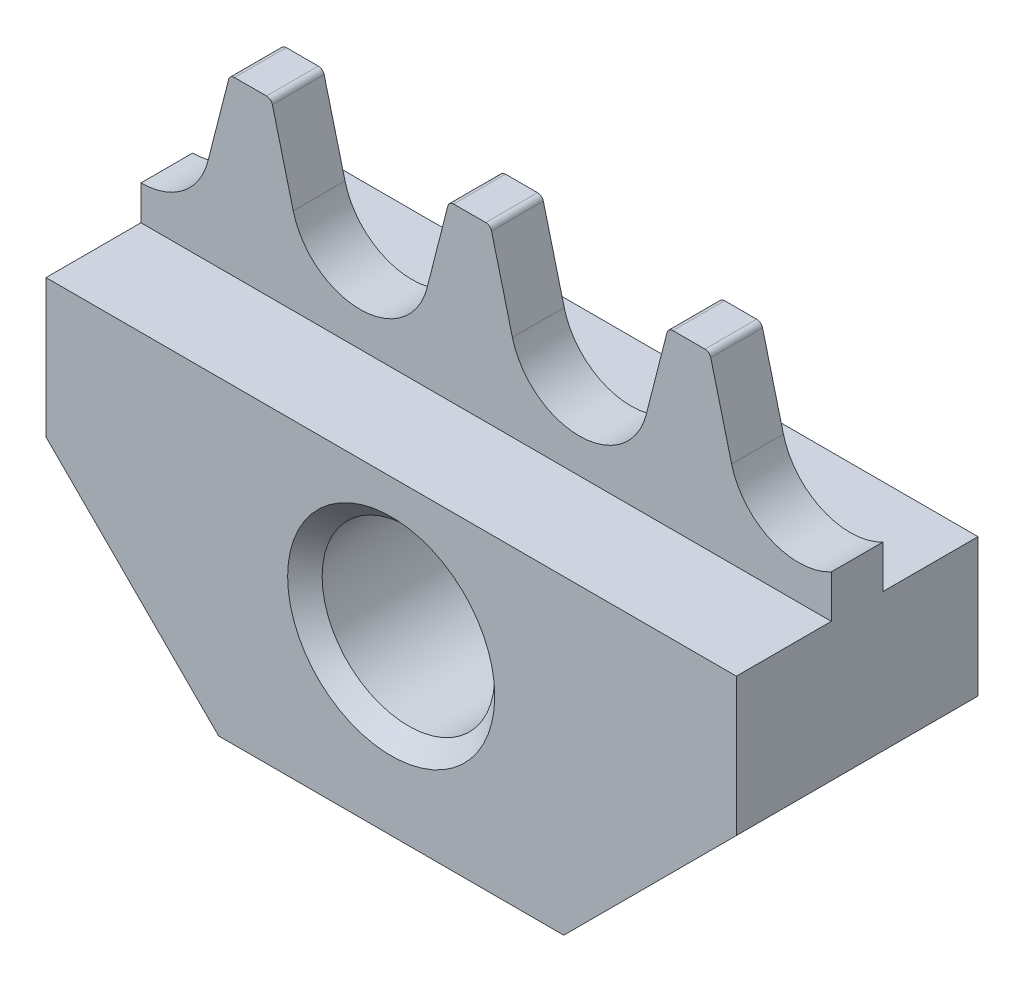
SolidWorks part; units mm, degrees
material "45"
ref_plane "前视基准面" through (0, 0, 0) normal (0, 0, 1) x (1, 0, 0)
ref_plane "上视基准面" through (0, 0, 0) normal (0, 1, 0) x (1, 0, 0)
ref_plane "右视基准面" through (0, 0, 0) normal (1, 0, 0) x (0, 0, -1)
sketch "草图1" plane through (0, 0, 0) normal (0, 0, 1) x (1, 0, 0)
  line L0 (0, 0) -> (0, 18) construction
  line L1 (20, 18) -> (-20, 18)
  line L2 (-20, 18) -> (-20, 10)
  line L4 (10, 0) -> (-10, 0)
  line L5 (-10, 0) -> (-20, 10)
  line L6 (10, 0) -> (20, 10)
  line L7 (20, 18) -> (20, 10)
  circle A0 centre (0, 10) radius 5
  dimension "D5" = 10
  dimension "D1" = 8
  dimension "D2" = 20
  dimension "D3" = 40
  dimension "D4" = 10
extrude "凸台-拉伸1" add sketch "草图1" along normal mid plane 14
sketch "草图2" plane through (0, 0, 0) normal (0, 0, 1) x (1, 0, 0)
  line L0 (-14.85, 28) -> (-12.45, 28)
  line L1 (-10, 0) -> (10, 0) construction
  line L2 (-20, 18) -> (-20, 10) construction
  line L3 (-35.3045, 24) -> (22.0082, 24) construction
  line L4 (-20, 24) -> (-7.3, 24) construction
  line L5 (-20, 18) -> (-20, 20)
  line L6 (-20, 18) -> (20, 18)
  line L7 (-14.85, 28) -> (-16.1244, 23.0102)
  line L8 (-13.65, 28) -> (-13.65, 18) construction
  line L9 (-12.45, 28) -> (-11.1756, 23.0102)
  line L10 (-2.15, 28) -> (-3.4244, 23.0102)
  line L11 (0.25, 28) -> (1.5244, 23.0102)
  line L12 (10.55, 28) -> (9.2756, 23.0102)
  line L13 (12.95, 28) -> (14.2244, 23.0102)
  line L14 (-14.85, 28) -> (-12.45, 28) construction
  line L15 (-2.15, 28) -> (0.25, 28)
  line L16 (10.55, 28) -> (12.95, 28)
  line L17 (20, 18) -> (20, 20.4801)
  arc A0 (-20, 20) -> (-16.1244, 23.0102) centre (-20, 24) ccw
  circle A1 centre (0, 10) radius 5 construction
  arc A2 (-11.1756, 23.0102) -> (-3.4244, 23.0102) centre (-7.3, 24) ccw
  arc A3 (1.5244, 23.0102) -> (9.2756, 23.0102) centre (5.4, 24) ccw
  arc A4 (14.2244, 23.0102) -> (20, 20.4801) centre (18.1, 24) ccw
  dimension "D1" = 8
  dimension "D2" = 28
  dimension "D3" = 14
  dimension "D4" = 4
  dimension "D6" = 6.35
  dimension "D7" = 2.4
extrude "凸台-拉伸2" add sketch "草图2" along normal mid plane 3
fillet "圆角1" radius 0.35 6 edges at (12.95, 28, 0) (10.55, 28, 0) (0.25, 28, 0) (-2.15, 28, 0) (-12.45, 28, 0) (-14.85, 28, 0)
chamfer "倒角1" distance 1 angle 45 2 edges at (5, 10, -7) (5, 10, 7)
